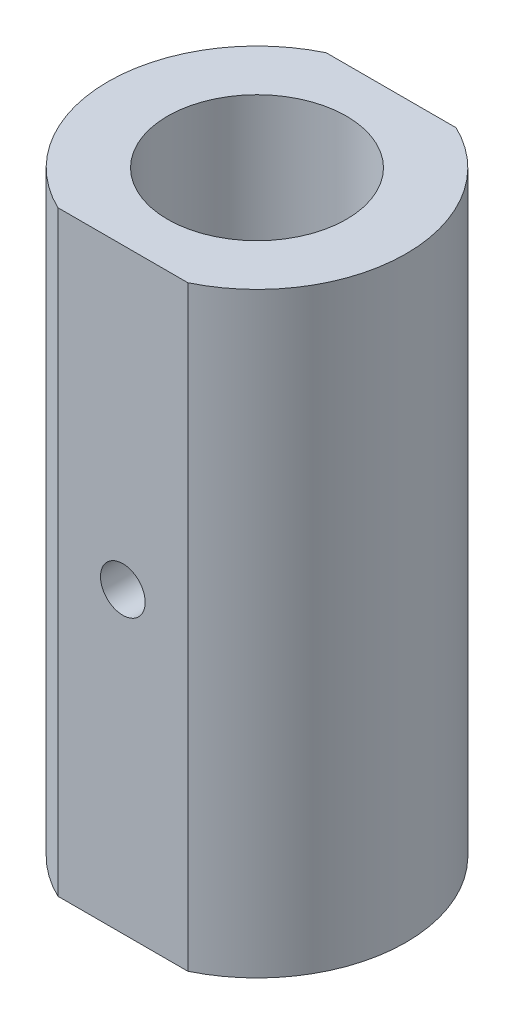
SolidWorks part; units mm, degrees
ref_plane "Front Plane" through (0, 0, 0) normal (0, 0, 1) x (1, 0, 0)
ref_plane "Top Plane" through (0, 0, 0) normal (0, 1, 0) x (1, 0, 0)
ref_plane "Right Plane" through (0, 0, 0) normal (1, 0, 0) x (0, 0, -1)
sketch "Sketch1" plane through (0, 0, 0) normal (0, 1, 0) x (1, 0, 0)
  line L0 (0, 0) -> (0, 0.4575)
  line L2 (2.1794, -4.5) -> (-2.1794, -4.5)
  line L3 (2.1794, 4.5) -> (-2.1794, 4.5)
  line L4 (0, 0.4575) -> (0, 0)
  arc A0 (-2.1794, 4.5) -> (-2.1794, -4.5) centre (0, 0) ccw
  circle A1 centre (0, 0) radius 3
  arc A2 (2.1794, -4.5) -> (2.1794, 4.5) centre (0, 0) ccw
  point P10 (0, -4.5)
  point P13 (0, 4.5)
  dimension "D1" = 10
  dimension "D2" = 6
  dimension "D3" = 4.5
  dimension "D4" = 4.5
  dimension "D5" = 9
extrude "Boss-Extrude1" add sketch "Sketch1" along normal blind 20 contours L2 A2 L3 A0 A1
sketch "Sketch2" plane through (0, 0, -4.5) normal (0, 0, -1) x (-1, 0, 0)
  line L0 (0, 20) -> (0, 0) construction
  line L1 (-2.1794, 20) -> (2.1794, 20) construction
  line L2 (-2.1794, 0) -> (2.1794, 0) construction
  circle A0 centre (0, 10) radius 0.75
  dimension "D1" = 1.5
extrude "Cut-Extrude1" cut sketch "Sketch2" against normal blind 20
